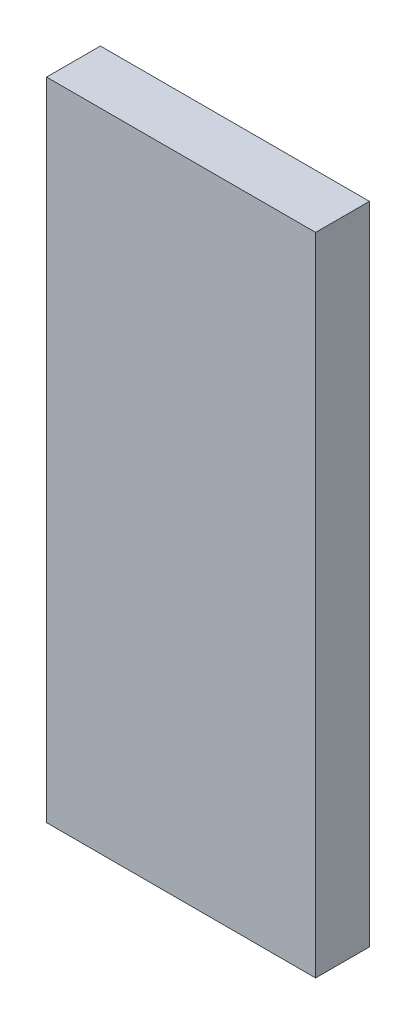
SolidWorks part; units mm, degrees
material "普通碳钢"
ref_plane "Front Plane" through (0, 0, 0) normal (0, 0, 1) x (1, 0, 0)
ref_plane "Top Plane" through (0, 0, 0) normal (0, 1, 0) x (1, 0, 0)
ref_plane "Right Plane" through (0, 0, 0) normal (1, 0, 0) x (0, 0, -1)
sketch "Sketch1" plane through (0, 0, 0) normal (0, 0, 1) x (1, 0, 0)
  line L1 (-25, 60) -> (25, 60)
  line L2 (-25, 60) -> (-25, -60)
  line L3 (-25, -60) -> (25, -60)
  line L4 (25, 60) -> (25, -60)
  dimension "D1" = 120
  dimension "D2" = 50
  dimension "D3" = 60
  dimension "D4" = 25
extrude "Boss-Extrude1" add sketch "Sketch1" along normal mid plane 10
